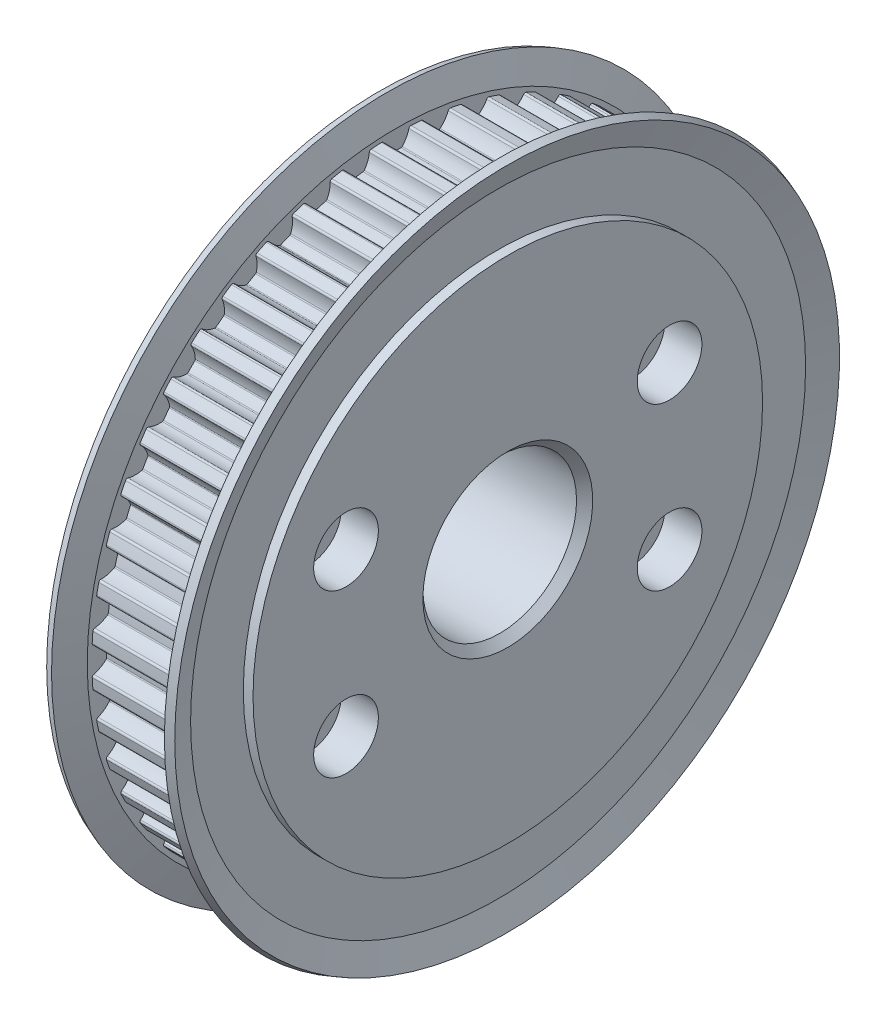
SolidWorks part; units mm, degrees
material "A7075"
ref_plane "Front Plane" through (0, 0, 0) normal (0, 0, 1) x (1, 0, 0)
ref_plane "Top Plane" through (0, 0, 0) normal (0, 1, 0) x (1, 0, 0)
ref_plane "Right Plane" through (0, 0, 0) normal (1, 0, 0) x (0, 0, -1)
sketch "Sketch1" plane through (0, 0, 0) normal (0, 0, 1) x (1, 0, 0)
  line L0 (0, 31.5) -> (0, 7.7)
  line L1 (0, 7.7) -> (0.2, 7.5)
  line L2 (0.2, 7.5) -> (27.8, 7.5)
  line L3 (27.8, 7.5) -> (28, 7.7)
  line L4 (28, 7.7) -> (28, 28.8)
  line L5 (28, 28.8) -> (27.8, 29)
  line L6 (27.8, 29) -> (16, 29)
  line L7 (16, 29) -> (16, 31.5)
  line L8 (16, 31.5) -> (14.8, 31.5)
  line L9 (14.8, 31.5) -> (14.8, 38.0191)
  line L10 (14.8, 38.0191) -> (15.9167, 41.0946)
  line L11 (15.9167, 41.0946) -> (14.9767, 41.4358)
  line L12 (14.9767, 41.4358) -> (13.8, 38.195)
  line L13 (13.8, 38.195) -> (2.2, 38.195)
  line L14 (2.2, 38.195) -> (1.0233, 41.4358)
  line L15 (1.0233, 41.4358) -> (0.0833, 41.0946)
  line L16 (0.0833, 41.0946) -> (1.2, 38.0191)
  line L17 (1.2, 38.0191) -> (1.2, 31.5)
  line L18 (1.2, 31.5) -> (0, 31.5)
  line L19 (28, 0) -> (0, 0) construction
revolve "Revolve1" add sketch "Sketch1" angle 360 about L19
sketch "Sketch2" plane through (0, 0, 0) normal (0, 0, 1) x (1, 0, 0)
  line L0 (16, 0) -> (16, 30)
  line L1 (16, 30) -> (28, 30)
  line L2 (28, 30) -> (28, 0)
  line L3 (28, 0) -> (16, 0)
  line L4 (28, 0) -> (16, 0) construction
revolve "Cut-Revolve1" cut sketch "Sketch2" angle 360 about L4
ref_plane "Plane1" through (2.2, 0, 0) normal (1, 0, 0) x (0, 0, -1)
sketch "Sketch3" plane through (2.2, 0, 0) normal (1, 0, 0) x (0, 0, -1)
  line L0 (-76.39, -76.39) -> (76.39, -76.39)
  line L1 (76.39, -76.39) -> (76.39, 76.39)
  line L2 (76.39, 76.39) -> (-76.39, 76.39)
  line L3 (-76.39, 76.39) -> (-76.39, -76.39)
  arc A0 (-37.5807, 1.8248) -> (-37.389, 1.5695) centre (-37.331, 1.8127) ccw
  arc A1 (-37.389, 1.5695) -> (-35.8722, 0.747) centre (-38.1589, -1.66) cw
  arc A2 (-35.8722, 0.747) -> (-35.81, 0.5986) centre (-36.01, 0.602) cw
  arc A3 (-35.81, 0.5986) -> (-35.81, -0.5986) centre (0, 0) ccw
  arc A4 (-35.81, -0.5986) -> (-35.8722, -0.747) centre (-36.01, -0.602) cw
  arc A5 (-35.8722, -0.747) -> (-37.389, -1.5695) centre (-38.1589, 1.66) cw
  arc A6 (-37.389, -1.5695) -> (-37.5807, -1.8248) centre (-37.331, -1.8127) ccw
  arc A7 (-37.5807, -1.8248) -> (-37.5444, -2.4608) centre (0, 0) ccw
  arc A8 (-37.5444, -2.4608) -> (-37.4974, -3.0961) centre (0, 0) ccw
  arc A9 (-37.4974, -3.0961) -> (-37.274, -3.3242) centre (-37.2482, -3.0755) ccw
  arc A10 (-37.274, -3.3242) -> (-35.6628, -3.9417) centre (-37.6158, -6.6265) cw
  arc A11 (-35.6628, -3.9417) -> (-35.5818, -4.0806) centre (-35.7805, -4.1034) cw
  arc A12 (-35.5818, -4.0806) -> (-35.4255, -5.2676) centre (0, 0) ccw
  arc A13 (-35.4255, -5.2676) -> (-35.4678, -5.4228) centre (-35.6233, -5.2971) cw
  arc A14 (-35.4678, -5.4228) -> (-36.8643, -6.4363) centre (-38.0491, -3.3349) cw
  arc A15 (-36.8643, -6.4363) -> (-37.021, -6.7145) centre (-36.775, -6.6698) ccw
  arc A16 (-37.021, -6.7145) -> (-36.902, -7.3403) centre (0, 0) ccw
  arc A17 (-36.902, -7.3403) -> (-36.7725, -7.964) centre (0, 0) ccw
  arc A18 (-36.7725, -7.964) -> (-36.5212, -8.161) centre (-36.5281, -7.9111) ccw
  arc A19 (-36.5212, -8.161) -> (-34.8432, -8.5629) centre (-36.429, -11.4797) cw
  arc A20 (-34.8432, -8.5629) -> (-34.7447, -8.6901) centre (-34.9388, -8.7386) cw
  arc A21 (-34.7447, -8.6901) -> (-34.4349, -9.8465) centre (0, 0) ccw
  arc A22 (-34.4349, -9.8465) -> (-34.4566, -10.0059) centre (-34.6272, -9.9015) cw
  arc A23 (-34.4566, -10.0059) -> (-35.7088, -11.193) centre (-37.2883, -8.2728) cw
  arc A24 (-35.7088, -11.193) -> (-35.8279, -11.4892) centre (-35.5898, -11.4129) ccw
  arc A25 (-35.8279, -11.4892) -> (-35.6282, -12.0942) centre (0, 0) ccw
  arc A26 (-35.6282, -12.0942) -> (-35.4184, -12.6956) centre (0, 0) ccw
  arc A27 (-35.4184, -12.6956) -> (-35.1435, -12.8581) centre (-35.183, -12.6113) ccw
  arc A28 (-35.1435, -12.8581) -> (-33.4275, -13.0376) centre (-34.619, -16.1364) cw
  arc A29 (-33.4275, -13.0376) -> (-33.3132, -13.1508) centre (-33.4992, -13.2243) cw
  arc A30 (-33.3132, -13.1508) -> (-32.855, -14.2569) centre (0, 0) ccw
  arc A31 (-32.855, -14.2569) -> (-32.8558, -14.4178) centre (-33.0385, -14.3366) cw
  arc A32 (-32.8558, -14.4178) -> (-33.9423, -15.7582) centre (-35.8895, -13.0691) cw
  arc A33 (-33.9423, -15.7582) -> (-34.0217, -16.0674) centre (-33.7957, -15.9607) ccw
  arc A34 (-34.0217, -16.0674) -> (-33.7448, -16.6411) centre (0, 0) ccw
  arc A35 (-33.7448, -16.6411) -> (-33.4583, -17.21) centre (0, 0) ccw
  arc A36 (-33.4583, -17.21) -> (-33.1646, -17.3353) centre (-33.2359, -17.0957) ccw
  arc A37 (-33.1646, -17.3353) -> (-31.4397, -17.2892) centre (-32.2166, -20.5171) cw
  arc A38 (-31.4397, -17.2892) -> (-31.3117, -17.3866) centre (-31.4865, -17.4837) cw
  arc A39 (-31.3117, -17.3866) -> (-30.7131, -18.4234) centre (0, 0) ccw
  arc A40 (-30.7131, -18.4234) -> (-30.6928, -18.583) centre (-30.8846, -18.5263) cw
  arc A41 (-30.6928, -18.583) -> (-31.5951, -20.0537) centre (-33.8766, -17.6419) cw
  arc A42 (-31.5951, -20.0537) -> (-31.6335, -20.3707) centre (-31.4233, -20.2353) ccw
  arc A43 (-31.6335, -20.3707) -> (-31.284, -20.9033) centre (0, 0) ccw
  arc A44 (-31.284, -20.9033) -> (-30.9257, -21.43) centre (0, 0) ccw
  arc A45 (-30.9257, -21.43) -> (-30.6181, -21.5158) centre (-30.7202, -21.2876) ccw
  arc A46 (-30.6181, -21.5158) -> (-28.9141, -21.245) centre (-29.263, -24.5466) cw
  arc A47 (-28.9141, -21.245) -> (-28.7744, -21.3248) centre (-28.9351, -21.4439) cw
  arc A48 (-28.7744, -21.3248) -> (-28.0456, -22.2747) centre (0, 0) ccw
  arc A49 (-28.0456, -22.2747) -> (-28.0046, -22.4302) centre (-28.2022, -22.399) cw
  arc A50 (-28.0046, -22.4302) -> (-28.7072, -24.0061) centre (-31.284, -21.9127) cw
  arc A51 (-28.7072, -24.0061) -> (-28.7039, -24.3254) centre (-28.5132, -24.1638) ccw
  arc A52 (-28.7039, -24.3254) -> (-28.288, -24.8079) centre (0, 0) ccw
  arc A53 (-28.288, -24.8079) -> (-27.8639, -25.2833) centre (0, 0) ccw
  arc A54 (-27.8639, -25.2833) -> (-27.5478, -25.3282) centre (-27.6788, -25.1153) ccw
  arc A55 (-27.5478, -25.3282) -> (-25.8937, -24.8373) centre (-25.8086, -28.1562) cw
  arc A56 (-25.8937, -24.8373) -> (-25.7448, -24.8982) centre (-25.8885, -25.0372) cw
  arc A57 (-25.7448, -24.8982) -> (-24.8982, -25.7448) centre (0, 0) ccw
  arc A58 (-24.8982, -25.7448) -> (-24.8373, -25.8937) centre (-25.0372, -25.8885) cw
  arc A59 (-24.8373, -25.8937) -> (-25.3282, -27.5478) centre (-28.1562, -25.8086) cw
  arc A60 (-25.3282, -27.5478) -> (-25.2833, -27.8639) centre (-25.1153, -27.6788) ccw
  arc A61 (-25.2833, -27.8639) -> (-24.8079, -28.288) centre (0, 0) ccw
  arc A62 (-24.8079, -28.288) -> (-24.3254, -28.7039) centre (0, 0) ccw
  arc A63 (-24.3254, -28.7039) -> (-24.0061, -28.7072) centre (-24.1638, -28.5132) ccw
  arc A64 (-24.0061, -28.7072) -> (-22.4302, -28.0046) centre (-21.9127, -31.284) cw
  arc A65 (-22.4302, -28.0046) -> (-22.2747, -28.0456) centre (-22.399, -28.2022) cw
  arc A66 (-22.2747, -28.0456) -> (-21.3248, -28.7744) centre (0, 0) ccw
  arc A67 (-21.3248, -28.7744) -> (-21.245, -28.9141) centre (-21.4439, -28.9351) cw
  arc A68 (-21.245, -28.9141) -> (-21.5158, -30.6181) centre (-24.5466, -29.263) cw
  arc A69 (-21.5158, -30.6181) -> (-21.43, -30.9257) centre (-21.2876, -30.7202) ccw
  arc A70 (-21.43, -30.9257) -> (-20.9033, -31.284) centre (0, 0) ccw
  arc A71 (-20.9033, -31.284) -> (-20.3707, -31.6335) centre (0, 0) ccw
  arc A72 (-20.3707, -31.6335) -> (-20.0537, -31.5951) centre (-20.2353, -31.4233) ccw
  arc A73 (-20.0537, -31.5951) -> (-18.583, -30.6928) centre (-17.6419, -33.8766) cw
  arc A74 (-18.583, -30.6928) -> (-18.4234, -30.7131) centre (-18.5263, -30.8846) cw
  arc A75 (-18.4234, -30.7131) -> (-17.3866, -31.3117) centre (0, 0) ccw
  arc A76 (-17.3866, -31.3117) -> (-17.2892, -31.4397) centre (-17.4837, -31.4865) cw
  arc A77 (-17.2892, -31.4397) -> (-17.3353, -33.1646) centre (-20.5171, -32.2166) cw
  arc A78 (-17.3353, -33.1646) -> (-17.21, -33.4583) centre (-17.0957, -33.2359) ccw
  arc A79 (-17.21, -33.4583) -> (-16.6411, -33.7448) centre (0, 0) ccw
  arc A80 (-16.6411, -33.7448) -> (-16.0674, -34.0217) centre (0, 0) ccw
  arc A81 (-16.0674, -34.0217) -> (-15.7582, -33.9423) centre (-15.9607, -33.7957) ccw
  arc A82 (-15.7582, -33.9423) -> (-14.4178, -32.8558) centre (-13.0691, -35.8895) cw
  arc A83 (-14.4178, -32.8558) -> (-14.2569, -32.855) centre (-14.3366, -33.0385) cw
  arc A84 (-14.2569, -32.855) -> (-13.1508, -33.3132) centre (0, 0) ccw
  arc A85 (-13.1508, -33.3132) -> (-13.0376, -33.4275) centre (-13.2243, -33.4992) cw
  arc A86 (-13.0376, -33.4275) -> (-12.8581, -35.1435) centre (-16.1364, -34.619) cw
  arc A87 (-12.8581, -35.1435) -> (-12.6956, -35.4184) centre (-12.6113, -35.183) ccw
  arc A88 (-12.6956, -35.4184) -> (-12.0942, -35.6282) centre (0, 0) ccw
  arc A89 (-12.0942, -35.6282) -> (-11.4892, -35.8279) centre (0, 0) ccw
  arc A90 (-11.4892, -35.8279) -> (-11.193, -35.7088) centre (-11.4129, -35.5898) ccw
  arc A91 (-11.193, -35.7088) -> (-10.0059, -34.4566) centre (-8.2728, -37.2883) cw
  arc A92 (-10.0059, -34.4566) -> (-9.8465, -34.4349) centre (-9.9015, -34.6272) cw
  arc A93 (-9.8465, -34.4349) -> (-8.6901, -34.7447) centre (0, 0) ccw
  arc A94 (-8.6901, -34.7447) -> (-8.5629, -34.8432) centre (-8.7386, -34.9388) cw
  arc A95 (-8.5629, -34.8432) -> (-8.161, -36.5212) centre (-11.4797, -36.429) cw
  arc A96 (-8.161, -36.5212) -> (-7.964, -36.7725) centre (-7.9111, -36.5281) ccw
  arc A97 (-7.964, -36.7725) -> (-7.3403, -36.902) centre (0, 0) ccw
  arc A98 (-7.3403, -36.902) -> (-6.7145, -37.021) centre (0, 0) ccw
  arc A99 (-6.7145, -37.021) -> (-6.4363, -36.8643) centre (-6.6698, -36.775) ccw
  arc A100 (-6.4363, -36.8643) -> (-5.4228, -35.4678) centre (-3.3349, -38.0491) cw
  arc A101 (-5.4228, -35.4678) -> (-5.2676, -35.4255) centre (-5.2971, -35.6233) cw
  arc A102 (-5.2676, -35.4255) -> (-4.0806, -35.5818) centre (0, 0) ccw
  arc A103 (-4.0806, -35.5818) -> (-3.9417, -35.6628) centre (-4.1034, -35.7805) cw
  arc A104 (-3.9417, -35.6628) -> (-3.3242, -37.274) centre (-6.6265, -37.6158) cw
  arc A105 (-3.3242, -37.274) -> (-3.0961, -37.4974) centre (-3.0755, -37.2482) ccw
  arc A106 (-3.0961, -37.4974) -> (-2.4608, -37.5444) centre (0, 0) ccw
  arc A107 (-2.4608, -37.5444) -> (-1.8248, -37.5807) centre (0, 0) ccw
  arc A108 (-1.8248, -37.5807) -> (-1.5695, -37.389) centre (-1.8127, -37.331) ccw
  arc A109 (-1.5695, -37.389) -> (-0.747, -35.8722) centre (1.66, -38.1589) cw
  arc A110 (-0.747, -35.8722) -> (-0.5986, -35.81) centre (-0.602, -36.01) cw
  arc A111 (-0.5986, -35.81) -> (0.5986, -35.81) centre (0, 0) ccw
  arc A112 (0.5986, -35.81) -> (0.747, -35.8722) centre (0.602, -36.01) cw
  arc A113 (0.747, -35.8722) -> (1.5695, -37.389) centre (-1.66, -38.1589) cw
  arc A114 (1.5695, -37.389) -> (1.8248, -37.5807) centre (1.8127, -37.331) ccw
  arc A115 (1.8248, -37.5807) -> (2.4608, -37.5444) centre (0, 0) ccw
  arc A116 (2.4608, -37.5444) -> (3.0961, -37.4974) centre (0, 0) ccw
  arc A117 (3.0961, -37.4974) -> (3.3242, -37.274) centre (3.0755, -37.2482) ccw
  arc A118 (3.3242, -37.274) -> (3.9417, -35.6628) centre (6.6265, -37.6158) cw
  arc A119 (3.9417, -35.6628) -> (4.0806, -35.5818) centre (4.1034, -35.7805) cw
  arc A120 (4.0806, -35.5818) -> (5.2676, -35.4255) centre (0, 0) ccw
  arc A121 (5.2676, -35.4255) -> (5.4228, -35.4678) centre (5.2971, -35.6233) cw
  arc A122 (5.4228, -35.4678) -> (6.4363, -36.8643) centre (3.3349, -38.0491) cw
  arc A123 (6.4363, -36.8643) -> (6.7145, -37.021) centre (6.6698, -36.775) ccw
  arc A124 (6.7145, -37.021) -> (7.3403, -36.902) centre (0, 0) ccw
  arc A125 (7.3403, -36.902) -> (7.964, -36.7725) centre (0, 0) ccw
  arc A126 (7.964, -36.7725) -> (8.161, -36.5212) centre (7.9111, -36.5281) ccw
  arc A127 (8.161, -36.5212) -> (8.5629, -34.8432) centre (11.4797, -36.429) cw
  arc A128 (8.5629, -34.8432) -> (8.6901, -34.7447) centre (8.7386, -34.9388) cw
  arc A129 (8.6901, -34.7447) -> (9.8465, -34.4349) centre (0, 0) ccw
  arc A130 (9.8465, -34.4349) -> (10.0059, -34.4566) centre (9.9015, -34.6272) cw
  arc A131 (10.0059, -34.4566) -> (11.193, -35.7088) centre (8.2728, -37.2883) cw
  arc A132 (11.193, -35.7088) -> (11.4892, -35.8279) centre (11.4129, -35.5898) ccw
  arc A133 (11.4892, -35.8279) -> (12.0942, -35.6282) centre (0, 0) ccw
  arc A134 (12.0942, -35.6282) -> (12.6956, -35.4184) centre (0, 0) ccw
  arc A135 (12.6956, -35.4184) -> (12.8581, -35.1435) centre (12.6113, -35.183) ccw
  arc A136 (12.8581, -35.1435) -> (13.0376, -33.4275) centre (16.1364, -34.619) cw
  arc A137 (13.0376, -33.4275) -> (13.1508, -33.3132) centre (13.2243, -33.4992) cw
  arc A138 (13.1508, -33.3132) -> (14.2569, -32.855) centre (0, 0) ccw
  arc A139 (14.2569, -32.855) -> (14.4178, -32.8558) centre (14.3366, -33.0385) cw
  arc A140 (14.4178, -32.8558) -> (15.7582, -33.9423) centre (13.0691, -35.8895) cw
  arc A141 (15.7582, -33.9423) -> (16.0674, -34.0217) centre (15.9607, -33.7957) ccw
  arc A142 (16.0674, -34.0217) -> (16.6411, -33.7448) centre (0, 0) ccw
  arc A143 (16.6411, -33.7448) -> (17.21, -33.4583) centre (0, 0) ccw
  arc A144 (17.21, -33.4583) -> (17.3353, -33.1646) centre (17.0957, -33.2359) ccw
  arc A145 (17.3353, -33.1646) -> (17.2892, -31.4397) centre (20.5171, -32.2166) cw
  arc A146 (17.2892, -31.4397) -> (17.3866, -31.3117) centre (17.4837, -31.4865) cw
  arc A147 (17.3866, -31.3117) -> (18.4234, -30.7131) centre (0, 0) ccw
  arc A148 (18.4234, -30.7131) -> (18.583, -30.6928) centre (18.5263, -30.8846) cw
  arc A149 (18.583, -30.6928) -> (20.0537, -31.5951) centre (17.6419, -33.8766) cw
  arc A150 (20.0537, -31.5951) -> (20.3707, -31.6335) centre (20.2353, -31.4233) ccw
  arc A151 (20.3707, -31.6335) -> (20.9033, -31.284) centre (0, 0) ccw
  arc A152 (20.9033, -31.284) -> (21.43, -30.9257) centre (0, 0) ccw
  arc A153 (21.43, -30.9257) -> (21.5158, -30.6181) centre (21.2876, -30.7202) ccw
  arc A154 (21.5158, -30.6181) -> (21.245, -28.9141) centre (24.5466, -29.263) cw
  arc A155 (21.245, -28.9141) -> (21.3248, -28.7744) centre (21.4439, -28.9351) cw
  arc A156 (21.3248, -28.7744) -> (22.2747, -28.0456) centre (0, 0) ccw
  arc A157 (22.2747, -28.0456) -> (22.4302, -28.0046) centre (22.399, -28.2022) cw
  arc A158 (22.4302, -28.0046) -> (24.0061, -28.7072) centre (21.9127, -31.284) cw
  arc A159 (24.0061, -28.7072) -> (24.3254, -28.7039) centre (24.1638, -28.5132) ccw
  arc A160 (24.3254, -28.7039) -> (24.8079, -28.288) centre (0, 0) ccw
  arc A161 (24.8079, -28.288) -> (25.2833, -27.8639) centre (0, 0) ccw
  arc A162 (25.2833, -27.8639) -> (25.3282, -27.5478) centre (25.1153, -27.6788) ccw
  arc A163 (25.3282, -27.5478) -> (24.8373, -25.8937) centre (28.1562, -25.8086) cw
  arc A164 (24.8373, -25.8937) -> (24.8982, -25.7448) centre (25.0372, -25.8885) cw
  arc A165 (24.8982, -25.7448) -> (25.7448, -24.8982) centre (0, 0) ccw
  arc A166 (25.7448, -24.8982) -> (25.8937, -24.8373) centre (25.8885, -25.0372) cw
  arc A167 (25.8937, -24.8373) -> (27.5478, -25.3282) centre (25.8086, -28.1562) cw
  arc A168 (27.5478, -25.3282) -> (27.8639, -25.2833) centre (27.6788, -25.1153) ccw
  arc A169 (27.8639, -25.2833) -> (28.288, -24.8079) centre (0, 0) ccw
  arc A170 (28.288, -24.8079) -> (28.7039, -24.3254) centre (0, 0) ccw
  arc A171 (28.7039, -24.3254) -> (28.7072, -24.0061) centre (28.5132, -24.1638) ccw
  arc A172 (28.7072, -24.0061) -> (28.0046, -22.4302) centre (31.284, -21.9127) cw
  arc A173 (28.0046, -22.4302) -> (28.0456, -22.2747) centre (28.2022, -22.399) cw
  arc A174 (28.0456, -22.2747) -> (28.7744, -21.3248) centre (0, 0) ccw
  arc A175 (28.7744, -21.3248) -> (28.9141, -21.245) centre (28.9351, -21.4439) cw
  arc A176 (28.9141, -21.245) -> (30.6181, -21.5158) centre (29.263, -24.5466) cw
  arc A177 (30.6181, -21.5158) -> (30.9257, -21.43) centre (30.7202, -21.2876) ccw
  arc A178 (30.9257, -21.43) -> (31.284, -20.9033) centre (0, 0) ccw
  arc A179 (31.284, -20.9033) -> (31.6335, -20.3707) centre (0, 0) ccw
  arc A180 (31.6335, -20.3707) -> (31.5951, -20.0537) centre (31.4233, -20.2353) ccw
  arc A181 (31.5951, -20.0537) -> (30.6928, -18.583) centre (33.8766, -17.6419) cw
  arc A182 (30.6928, -18.583) -> (30.7131, -18.4234) centre (30.8846, -18.5263) cw
  arc A183 (30.7131, -18.4234) -> (31.3117, -17.3866) centre (0, 0) ccw
  arc A184 (31.3117, -17.3866) -> (31.4397, -17.2892) centre (31.4865, -17.4837) cw
  arc A185 (31.4397, -17.2892) -> (33.1646, -17.3353) centre (32.2166, -20.5171) cw
  arc A186 (33.1646, -17.3353) -> (33.4583, -17.21) centre (33.2359, -17.0957) ccw
  arc A187 (33.4583, -17.21) -> (33.7448, -16.6411) centre (0, 0) ccw
  arc A188 (33.7448, -16.6411) -> (34.0217, -16.0674) centre (0, 0) ccw
  arc A189 (34.0217, -16.0674) -> (33.9423, -15.7582) centre (33.7957, -15.9607) ccw
  arc A190 (33.9423, -15.7582) -> (32.8558, -14.4178) centre (35.8895, -13.0691) cw
  arc A191 (32.8558, -14.4178) -> (32.855, -14.2569) centre (33.0385, -14.3366) cw
  arc A192 (32.855, -14.2569) -> (33.3132, -13.1508) centre (0, 0) ccw
  arc A193 (33.3132, -13.1508) -> (33.4275, -13.0376) centre (33.4992, -13.2243) cw
  arc A194 (33.4275, -13.0376) -> (35.1435, -12.8581) centre (34.619, -16.1364) cw
  arc A195 (35.1435, -12.8581) -> (35.4184, -12.6956) centre (35.183, -12.6113) ccw
  arc A196 (35.4184, -12.6956) -> (35.6282, -12.0942) centre (0, 0) ccw
  arc A197 (35.6282, -12.0942) -> (35.8279, -11.4892) centre (0, 0) ccw
  arc A198 (35.8279, -11.4892) -> (35.7088, -11.193) centre (35.5898, -11.4129) ccw
  arc A199 (35.7088, -11.193) -> (34.4566, -10.0059) centre (37.2883, -8.2728) cw
  arc A200 (34.4566, -10.0059) -> (34.4349, -9.8465) centre (34.6272, -9.9015) cw
  arc A201 (34.4349, -9.8465) -> (34.7447, -8.6901) centre (0, 0) ccw
  arc A202 (34.7447, -8.6901) -> (34.8432, -8.5629) centre (34.9388, -8.7386) cw
  arc A203 (34.8432, -8.5629) -> (36.5212, -8.161) centre (36.429, -11.4797) cw
  arc A204 (36.5212, -8.161) -> (36.7725, -7.964) centre (36.5281, -7.9111) ccw
  arc A205 (36.7725, -7.964) -> (36.902, -7.3403) centre (0, 0) ccw
  arc A206 (36.902, -7.3403) -> (37.021, -6.7145) centre (0, 0) ccw
  arc A207 (37.021, -6.7145) -> (36.8643, -6.4363) centre (36.775, -6.6698) ccw
  arc A208 (36.8643, -6.4363) -> (35.4678, -5.4228) centre (38.0491, -3.3349) cw
  arc A209 (35.4678, -5.4228) -> (35.4255, -5.2676) centre (35.6233, -5.2971) cw
  arc A210 (35.4255, -5.2676) -> (35.5818, -4.0806) centre (0, 0) ccw
  arc A211 (35.5818, -4.0806) -> (35.6628, -3.9417) centre (35.7805, -4.1034) cw
  arc A212 (35.6628, -3.9417) -> (37.274, -3.3242) centre (37.6158, -6.6265) cw
  arc A213 (37.274, -3.3242) -> (37.4974, -3.0961) centre (37.2482, -3.0755) ccw
  arc A214 (37.4974, -3.0961) -> (37.5444, -2.4608) centre (0, 0) ccw
  arc A215 (37.5444, -2.4608) -> (37.5807, -1.8248) centre (0, 0) ccw
  arc A216 (37.5807, -1.8248) -> (37.389, -1.5695) centre (37.331, -1.8127) ccw
  arc A217 (37.389, -1.5695) -> (35.8722, -0.747) centre (38.1589, 1.66) cw
  arc A218 (35.8722, -0.747) -> (35.81, -0.5986) centre (36.01, -0.602) cw
  arc A219 (35.81, -0.5986) -> (35.81, 0.5986) centre (0, 0) ccw
  arc A220 (35.81, 0.5986) -> (35.8722, 0.747) centre (36.01, 0.602) cw
  arc A221 (35.8722, 0.747) -> (37.389, 1.5695) centre (38.1589, -1.66) cw
  arc A222 (37.389, 1.5695) -> (37.5807, 1.8248) centre (37.331, 1.8127) ccw
  arc A223 (37.5807, 1.8248) -> (37.5444, 2.4608) centre (0, 0) ccw
  arc A224 (37.5444, 2.4608) -> (37.4974, 3.0961) centre (0, 0) ccw
  arc A225 (37.4974, 3.0961) -> (37.274, 3.3242) centre (37.2482, 3.0755) ccw
  arc A226 (37.274, 3.3242) -> (35.6628, 3.9417) centre (37.6158, 6.6265) cw
  arc A227 (35.6628, 3.9417) -> (35.5818, 4.0806) centre (35.7805, 4.1034) cw
  arc A228 (35.5818, 4.0806) -> (35.4255, 5.2676) centre (0, 0) ccw
  arc A229 (35.4255, 5.2676) -> (35.4678, 5.4228) centre (35.6233, 5.2971) cw
  arc A230 (35.4678, 5.4228) -> (36.8643, 6.4363) centre (38.0491, 3.3349) cw
  arc A231 (36.8643, 6.4363) -> (37.021, 6.7145) centre (36.775, 6.6698) ccw
  arc A232 (37.021, 6.7145) -> (36.902, 7.3403) centre (0, 0) ccw
  arc A233 (36.902, 7.3403) -> (36.7725, 7.964) centre (0, 0) ccw
  arc A234 (36.7725, 7.964) -> (36.5212, 8.161) centre (36.5281, 7.9111) ccw
  arc A235 (36.5212, 8.161) -> (34.8432, 8.5629) centre (36.429, 11.4797) cw
  arc A236 (34.8432, 8.5629) -> (34.7447, 8.6901) centre (34.9388, 8.7386) cw
  arc A237 (34.7447, 8.6901) -> (34.4349, 9.8465) centre (0, 0) ccw
  arc A238 (34.4349, 9.8465) -> (34.4566, 10.0059) centre (34.6272, 9.9015) cw
  arc A239 (34.4566, 10.0059) -> (35.7088, 11.193) centre (37.2883, 8.2728) cw
  arc A240 (35.7088, 11.193) -> (35.8279, 11.4892) centre (35.5898, 11.4129) ccw
  arc A241 (35.8279, 11.4892) -> (35.6282, 12.0942) centre (0, 0) ccw
  arc A242 (35.6282, 12.0942) -> (35.4184, 12.6956) centre (0, 0) ccw
  arc A243 (35.4184, 12.6956) -> (35.1435, 12.8581) centre (35.183, 12.6113) ccw
  arc A244 (35.1435, 12.8581) -> (33.4275, 13.0376) centre (34.619, 16.1364) cw
  arc A245 (33.4275, 13.0376) -> (33.3132, 13.1508) centre (33.4992, 13.2243) cw
  arc A246 (33.3132, 13.1508) -> (32.855, 14.2569) centre (0, 0) ccw
  arc A247 (32.855, 14.2569) -> (32.8558, 14.4178) centre (33.0385, 14.3366) cw
  arc A248 (32.8558, 14.4178) -> (33.9423, 15.7582) centre (35.8895, 13.0691) cw
  arc A249 (33.9423, 15.7582) -> (34.0217, 16.0674) centre (33.7957, 15.9607) ccw
  arc A250 (34.0217, 16.0674) -> (33.7448, 16.6411) centre (0, 0) ccw
  arc A251 (33.7448, 16.6411) -> (33.4583, 17.21) centre (0, 0) ccw
  arc A252 (33.4583, 17.21) -> (33.1646, 17.3353) centre (33.2359, 17.0957) ccw
  arc A253 (33.1646, 17.3353) -> (31.4397, 17.2892) centre (32.2166, 20.5171) cw
  arc A254 (31.4397, 17.2892) -> (31.3117, 17.3866) centre (31.4865, 17.4837) cw
  arc A255 (31.3117, 17.3866) -> (30.7131, 18.4234) centre (0, 0) ccw
  arc A256 (30.7131, 18.4234) -> (30.6928, 18.583) centre (30.8846, 18.5263) cw
  arc A257 (30.6928, 18.583) -> (31.5951, 20.0537) centre (33.8766, 17.6419) cw
  arc A258 (31.5951, 20.0537) -> (31.6335, 20.3707) centre (31.4233, 20.2353) ccw
  arc A259 (31.6335, 20.3707) -> (31.284, 20.9033) centre (0, 0) ccw
  arc A260 (31.284, 20.9033) -> (30.9257, 21.43) centre (0, 0) ccw
  arc A261 (30.9257, 21.43) -> (30.6181, 21.5158) centre (30.7202, 21.2876) ccw
  arc A262 (30.6181, 21.5158) -> (28.9141, 21.245) centre (29.263, 24.5466) cw
  arc A263 (28.9141, 21.245) -> (28.7744, 21.3248) centre (28.9351, 21.4439) cw
  arc A264 (28.7744, 21.3248) -> (28.0456, 22.2747) centre (0, 0) ccw
  arc A265 (28.0456, 22.2747) -> (28.0046, 22.4302) centre (28.2022, 22.399) cw
  arc A266 (28.0046, 22.4302) -> (28.7072, 24.0061) centre (31.284, 21.9127) cw
  arc A267 (28.7072, 24.0061) -> (28.7039, 24.3254) centre (28.5132, 24.1638) ccw
  arc A268 (28.7039, 24.3254) -> (28.288, 24.8079) centre (0, 0) ccw
  arc A269 (28.288, 24.8079) -> (27.8639, 25.2833) centre (0, 0) ccw
  arc A270 (27.8639, 25.2833) -> (27.5478, 25.3282) centre (27.6788, 25.1153) ccw
  arc A271 (27.5478, 25.3282) -> (25.8937, 24.8373) centre (25.8086, 28.1562) cw
  arc A272 (25.8937, 24.8373) -> (25.7448, 24.8982) centre (25.8885, 25.0372) cw
  arc A273 (25.7448, 24.8982) -> (24.8982, 25.7448) centre (0, 0) ccw
  arc A274 (24.8982, 25.7448) -> (24.8373, 25.8937) centre (25.0372, 25.8885) cw
  arc A275 (24.8373, 25.8937) -> (25.3282, 27.5478) centre (28.1562, 25.8086) cw
  arc A276 (25.3282, 27.5478) -> (25.2833, 27.8639) centre (25.1153, 27.6788) ccw
  arc A277 (25.2833, 27.8639) -> (24.8079, 28.288) centre (0, 0) ccw
  arc A278 (24.8079, 28.288) -> (24.3254, 28.7039) centre (0, 0) ccw
  arc A279 (24.3254, 28.7039) -> (24.0061, 28.7072) centre (24.1638, 28.5132) ccw
  arc A280 (24.0061, 28.7072) -> (22.4302, 28.0046) centre (21.9127, 31.284) cw
  arc A281 (22.4302, 28.0046) -> (22.2747, 28.0456) centre (22.399, 28.2022) cw
  arc A282 (22.2747, 28.0456) -> (21.3248, 28.7744) centre (0, 0) ccw
  arc A283 (21.3248, 28.7744) -> (21.245, 28.9141) centre (21.4439, 28.9351) cw
  arc A284 (21.245, 28.9141) -> (21.5158, 30.6181) centre (24.5466, 29.263) cw
  arc A285 (21.5158, 30.6181) -> (21.43, 30.9257) centre (21.2876, 30.7202) ccw
  arc A286 (21.43, 30.9257) -> (20.9033, 31.284) centre (0, 0) ccw
  arc A287 (20.9033, 31.284) -> (20.3707, 31.6335) centre (0, 0) ccw
  arc A288 (20.3707, 31.6335) -> (20.0537, 31.5951) centre (20.2353, 31.4233) ccw
  arc A289 (20.0537, 31.5951) -> (18.583, 30.6928) centre (17.6419, 33.8766) cw
  arc A290 (18.583, 30.6928) -> (18.4234, 30.7131) centre (18.5263, 30.8846) cw
  arc A291 (18.4234, 30.7131) -> (17.3866, 31.3117) centre (0, 0) ccw
  arc A292 (17.3866, 31.3117) -> (17.2892, 31.4397) centre (17.4837, 31.4865) cw
  arc A293 (17.2892, 31.4397) -> (17.3353, 33.1646) centre (20.5171, 32.2166) cw
  arc A294 (17.3353, 33.1646) -> (17.21, 33.4583) centre (17.0957, 33.2359) ccw
  arc A295 (17.21, 33.4583) -> (16.6411, 33.7448) centre (0, 0) ccw
  arc A296 (16.6411, 33.7448) -> (16.0674, 34.0217) centre (0, 0) ccw
  arc A297 (16.0674, 34.0217) -> (15.7582, 33.9423) centre (15.9607, 33.7957) ccw
  arc A298 (15.7582, 33.9423) -> (14.4178, 32.8558) centre (13.0691, 35.8895) cw
  arc A299 (14.4178, 32.8558) -> (14.2569, 32.855) centre (14.3366, 33.0385) cw
  arc A300 (14.2569, 32.855) -> (13.1508, 33.3132) centre (0, 0) ccw
  arc A301 (13.1508, 33.3132) -> (13.0376, 33.4275) centre (13.2243, 33.4992) cw
  arc A302 (13.0376, 33.4275) -> (12.8581, 35.1435) centre (16.1364, 34.619) cw
  arc A303 (12.8581, 35.1435) -> (12.6956, 35.4184) centre (12.6113, 35.183) ccw
  arc A304 (12.6956, 35.4184) -> (12.0942, 35.6282) centre (0, 0) ccw
  arc A305 (12.0942, 35.6282) -> (11.4892, 35.8279) centre (0, 0) ccw
  arc A306 (11.4892, 35.8279) -> (11.193, 35.7088) centre (11.4129, 35.5898) ccw
  arc A307 (11.193, 35.7088) -> (10.0059, 34.4566) centre (8.2728, 37.2883) cw
  arc A308 (10.0059, 34.4566) -> (9.8465, 34.4349) centre (9.9015, 34.6272) cw
  arc A309 (9.8465, 34.4349) -> (8.6901, 34.7447) centre (0, 0) ccw
  arc A310 (8.6901, 34.7447) -> (8.5629, 34.8432) centre (8.7386, 34.9388) cw
  arc A311 (8.5629, 34.8432) -> (8.161, 36.5212) centre (11.4797, 36.429) cw
  arc A312 (8.161, 36.5212) -> (7.964, 36.7725) centre (7.9111, 36.5281) ccw
  arc A313 (7.964, 36.7725) -> (7.3403, 36.902) centre (0, 0) ccw
  arc A314 (7.3403, 36.902) -> (6.7145, 37.021) centre (0, 0) ccw
  arc A315 (6.7145, 37.021) -> (6.4363, 36.8643) centre (6.6698, 36.775) ccw
  arc A316 (6.4363, 36.8643) -> (5.4228, 35.4678) centre (3.3349, 38.0491) cw
  arc A317 (5.4228, 35.4678) -> (5.2676, 35.4255) centre (5.2971, 35.6233) cw
  arc A318 (5.2676, 35.4255) -> (4.0806, 35.5818) centre (0, 0) ccw
  arc A319 (4.0806, 35.5818) -> (3.9417, 35.6628) centre (4.1034, 35.7805) cw
  arc A320 (3.9417, 35.6628) -> (3.3242, 37.274) centre (6.6265, 37.6158) cw
  arc A321 (3.3242, 37.274) -> (3.0961, 37.4974) centre (3.0755, 37.2482) ccw
  arc A322 (3.0961, 37.4974) -> (2.4608, 37.5444) centre (0, 0) ccw
  arc A323 (2.4608, 37.5444) -> (1.8248, 37.5807) centre (0, 0) ccw
  arc A324 (1.8248, 37.5807) -> (1.5695, 37.389) centre (1.8127, 37.331) ccw
  arc A325 (1.5695, 37.389) -> (0.747, 35.8722) centre (-1.66, 38.1589) cw
  arc A326 (0.747, 35.8722) -> (0.5986, 35.81) centre (0.602, 36.01) cw
  arc A327 (0.5986, 35.81) -> (-0.5986, 35.81) centre (0, 0) ccw
  arc A328 (-0.5986, 35.81) -> (-0.747, 35.8722) centre (-0.602, 36.01) cw
  arc A329 (-0.747, 35.8722) -> (-1.5695, 37.389) centre (1.66, 38.1589) cw
  arc A330 (-1.5695, 37.389) -> (-1.8248, 37.5807) centre (-1.8127, 37.331) ccw
  arc A331 (-1.8248, 37.5807) -> (-2.4608, 37.5444) centre (0, 0) ccw
  arc A332 (-2.4608, 37.5444) -> (-3.0961, 37.4974) centre (0, 0) ccw
  arc A333 (-3.0961, 37.4974) -> (-3.3242, 37.274) centre (-3.0755, 37.2482) ccw
  arc A334 (-3.3242, 37.274) -> (-3.9417, 35.6628) centre (-6.6265, 37.6158) cw
  arc A335 (-3.9417, 35.6628) -> (-4.0806, 35.5818) centre (-4.1034, 35.7805) cw
  arc A336 (-4.0806, 35.5818) -> (-5.2676, 35.4255) centre (0, 0) ccw
  arc A337 (-5.2676, 35.4255) -> (-5.4228, 35.4678) centre (-5.2971, 35.6233) cw
  arc A338 (-5.4228, 35.4678) -> (-6.4363, 36.8643) centre (-3.3349, 38.0491) cw
  arc A339 (-6.4363, 36.8643) -> (-6.7145, 37.021) centre (-6.6698, 36.775) ccw
  arc A340 (-6.7145, 37.021) -> (-7.3403, 36.902) centre (0, 0) ccw
  arc A341 (-7.3403, 36.902) -> (-7.964, 36.7725) centre (0, 0) ccw
  arc A342 (-7.964, 36.7725) -> (-8.161, 36.5212) centre (-7.9111, 36.5281) ccw
  arc A343 (-8.161, 36.5212) -> (-8.5629, 34.8432) centre (-11.4797, 36.429) cw
  arc A344 (-8.5629, 34.8432) -> (-8.6901, 34.7447) centre (-8.7386, 34.9388) cw
  arc A345 (-8.6901, 34.7447) -> (-9.8465, 34.4349) centre (0, 0) ccw
  arc A346 (-9.8465, 34.4349) -> (-10.0059, 34.4566) centre (-9.9015, 34.6272) cw
  arc A347 (-10.0059, 34.4566) -> (-11.193, 35.7088) centre (-8.2728, 37.2883) cw
  arc A348 (-11.193, 35.7088) -> (-11.4892, 35.8279) centre (-11.4129, 35.5898) ccw
  arc A349 (-11.4892, 35.8279) -> (-12.0942, 35.6282) centre (0, 0) ccw
  arc A350 (-12.0942, 35.6282) -> (-12.6956, 35.4184) centre (0, 0) ccw
  arc A351 (-12.6956, 35.4184) -> (-12.8581, 35.1435) centre (-12.6113, 35.183) ccw
  arc A352 (-12.8581, 35.1435) -> (-13.0376, 33.4275) centre (-16.1364, 34.619) cw
  arc A353 (-13.0376, 33.4275) -> (-13.1508, 33.3132) centre (-13.2243, 33.4992) cw
  arc A354 (-13.1508, 33.3132) -> (-14.2569, 32.855) centre (0, 0) ccw
  arc A355 (-14.2569, 32.855) -> (-14.4178, 32.8558) centre (-14.3366, 33.0385) cw
  arc A356 (-14.4178, 32.8558) -> (-15.7582, 33.9423) centre (-13.0691, 35.8895) cw
  arc A357 (-15.7582, 33.9423) -> (-16.0674, 34.0217) centre (-15.9607, 33.7957) ccw
  arc A358 (-16.0674, 34.0217) -> (-16.6411, 33.7448) centre (0, 0) ccw
  arc A359 (-16.6411, 33.7448) -> (-17.21, 33.4583) centre (0, 0) ccw
  arc A360 (-17.21, 33.4583) -> (-17.3353, 33.1646) centre (-17.0957, 33.2359) ccw
  arc A361 (-17.3353, 33.1646) -> (-17.2892, 31.4397) centre (-20.5171, 32.2166) cw
  arc A362 (-17.2892, 31.4397) -> (-17.3866, 31.3117) centre (-17.4837, 31.4865) cw
  arc A363 (-17.3866, 31.3117) -> (-18.4234, 30.7131) centre (0, 0) ccw
  arc A364 (-18.4234, 30.7131) -> (-18.583, 30.6928) centre (-18.5263, 30.8846) cw
  arc A365 (-18.583, 30.6928) -> (-20.0537, 31.5951) centre (-17.6419, 33.8766) cw
  arc A366 (-20.0537, 31.5951) -> (-20.3707, 31.6335) centre (-20.2353, 31.4233) ccw
  arc A367 (-20.3707, 31.6335) -> (-20.9033, 31.284) centre (0, 0) ccw
  arc A368 (-20.9033, 31.284) -> (-21.43, 30.9257) centre (0, 0) ccw
  arc A369 (-21.43, 30.9257) -> (-21.5158, 30.6181) centre (-21.2876, 30.7202) ccw
  arc A370 (-21.5158, 30.6181) -> (-21.245, 28.9141) centre (-24.5466, 29.263) cw
  arc A371 (-21.245, 28.9141) -> (-21.3248, 28.7744) centre (-21.4439, 28.9351) cw
  arc A372 (-21.3248, 28.7744) -> (-22.2747, 28.0456) centre (0, 0) ccw
  arc A373 (-22.2747, 28.0456) -> (-22.4302, 28.0046) centre (-22.399, 28.2022) cw
  arc A374 (-22.4302, 28.0046) -> (-24.0061, 28.7072) centre (-21.9127, 31.284) cw
  arc A375 (-24.0061, 28.7072) -> (-24.3254, 28.7039) centre (-24.1638, 28.5132) ccw
  arc A376 (-24.3254, 28.7039) -> (-24.8079, 28.288) centre (0, 0) ccw
  arc A377 (-24.8079, 28.288) -> (-25.2833, 27.8639) centre (0, 0) ccw
  arc A378 (-25.2833, 27.8639) -> (-25.3282, 27.5478) centre (-25.1153, 27.6788) ccw
  arc A379 (-25.3282, 27.5478) -> (-24.8373, 25.8937) centre (-28.1562, 25.8086) cw
  arc A380 (-24.8373, 25.8937) -> (-24.8982, 25.7448) centre (-25.0372, 25.8885) cw
  arc A381 (-24.8982, 25.7448) -> (-25.7448, 24.8982) centre (0, 0) ccw
  arc A382 (-25.7448, 24.8982) -> (-25.8937, 24.8373) centre (-25.8885, 25.0372) cw
  arc A383 (-25.8937, 24.8373) -> (-27.5478, 25.3282) centre (-25.8086, 28.1562) cw
  arc A384 (-27.5478, 25.3282) -> (-27.8639, 25.2833) centre (-27.6788, 25.1153) ccw
  arc A385 (-27.8639, 25.2833) -> (-28.288, 24.8079) centre (0, 0) ccw
  arc A386 (-28.288, 24.8079) -> (-28.7039, 24.3254) centre (0, 0) ccw
  arc A387 (-28.7039, 24.3254) -> (-28.7072, 24.0061) centre (-28.5132, 24.1638) ccw
  arc A388 (-28.7072, 24.0061) -> (-28.0046, 22.4302) centre (-31.284, 21.9127) cw
  arc A389 (-28.0046, 22.4302) -> (-28.0456, 22.2747) centre (-28.2022, 22.399) cw
  arc A390 (-28.0456, 22.2747) -> (-28.7744, 21.3248) centre (0, 0) ccw
  arc A391 (-28.7744, 21.3248) -> (-28.9141, 21.245) centre (-28.9351, 21.4439) cw
  arc A392 (-28.9141, 21.245) -> (-30.6181, 21.5158) centre (-29.263, 24.5466) cw
  arc A393 (-30.6181, 21.5158) -> (-30.9257, 21.43) centre (-30.7202, 21.2876) ccw
  arc A394 (-30.9257, 21.43) -> (-31.284, 20.9033) centre (0, 0) ccw
  arc A395 (-31.284, 20.9033) -> (-31.6335, 20.3707) centre (0, 0) ccw
  arc A396 (-31.6335, 20.3707) -> (-31.5951, 20.0537) centre (-31.4233, 20.2353) ccw
  arc A397 (-31.5951, 20.0537) -> (-30.6928, 18.583) centre (-33.8766, 17.6419) cw
  arc A398 (-30.6928, 18.583) -> (-30.7131, 18.4234) centre (-30.8846, 18.5263) cw
  arc A399 (-30.7131, 18.4234) -> (-31.3117, 17.3866) centre (0, 0) ccw
  arc A400 (-31.3117, 17.3866) -> (-31.4397, 17.2892) centre (-31.4865, 17.4837) cw
  arc A401 (-31.4397, 17.2892) -> (-33.1646, 17.3353) centre (-32.2166, 20.5171) cw
  arc A402 (-33.1646, 17.3353) -> (-33.4583, 17.21) centre (-33.2359, 17.0957) ccw
  arc A403 (-33.4583, 17.21) -> (-33.7448, 16.6411) centre (0, 0) ccw
  arc A404 (-33.7448, 16.6411) -> (-34.0217, 16.0674) centre (0, 0) ccw
  arc A405 (-34.0217, 16.0674) -> (-33.9423, 15.7582) centre (-33.7957, 15.9607) ccw
  arc A406 (-33.9423, 15.7582) -> (-32.8558, 14.4178) centre (-35.8895, 13.0691) cw
  arc A407 (-32.8558, 14.4178) -> (-32.855, 14.2569) centre (-33.0385, 14.3366) cw
  arc A408 (-32.855, 14.2569) -> (-33.3132, 13.1508) centre (0, 0) ccw
  arc A409 (-33.3132, 13.1508) -> (-33.4275, 13.0376) centre (-33.4992, 13.2243) cw
  arc A410 (-33.4275, 13.0376) -> (-35.1435, 12.8581) centre (-34.619, 16.1364) cw
  arc A411 (-35.1435, 12.8581) -> (-35.4184, 12.6956) centre (-35.183, 12.6113) ccw
  arc A412 (-35.4184, 12.6956) -> (-35.6282, 12.0942) centre (0, 0) ccw
  arc A413 (-35.6282, 12.0942) -> (-35.8279, 11.4892) centre (0, 0) ccw
  arc A414 (-35.8279, 11.4892) -> (-35.7088, 11.193) centre (-35.5898, 11.4129) ccw
  arc A415 (-35.7088, 11.193) -> (-34.4566, 10.0059) centre (-37.2883, 8.2728) cw
  arc A416 (-34.4566, 10.0059) -> (-34.4349, 9.8465) centre (-34.6272, 9.9015) cw
  arc A417 (-34.4349, 9.8465) -> (-34.7447, 8.6901) centre (0, 0) ccw
  arc A418 (-34.7447, 8.6901) -> (-34.8432, 8.5629) centre (-34.9388, 8.7386) cw
  arc A419 (-34.8432, 8.5629) -> (-36.5212, 8.161) centre (-36.429, 11.4797) cw
  arc A420 (-36.5212, 8.161) -> (-36.7725, 7.964) centre (-36.5281, 7.9111) ccw
  arc A421 (-36.7725, 7.964) -> (-36.902, 7.3403) centre (0, 0) ccw
  arc A422 (-36.902, 7.3403) -> (-37.021, 6.7145) centre (0, 0) ccw
  arc A423 (-37.021, 6.7145) -> (-36.8643, 6.4363) centre (-36.775, 6.6698) ccw
  arc A424 (-36.8643, 6.4363) -> (-35.4678, 5.4228) centre (-38.0491, 3.3349) cw
  arc A425 (-35.4678, 5.4228) -> (-35.4255, 5.2676) centre (-35.6233, 5.2971) cw
  arc A426 (-35.4255, 5.2676) -> (-35.5818, 4.0806) centre (0, 0) ccw
  arc A427 (-35.5818, 4.0806) -> (-35.6628, 3.9417) centre (-35.7805, 4.1034) cw
  arc A428 (-35.6628, 3.9417) -> (-37.274, 3.3242) centre (-37.6158, 6.6265) cw
  arc A429 (-37.274, 3.3242) -> (-37.4974, 3.0961) centre (-37.2482, 3.0755) ccw
  arc A430 (-37.4974, 3.0961) -> (-37.5444, 2.4608) centre (0, 0) ccw
  arc A431 (-37.5444, 2.4608) -> (-37.5807, 1.8248) centre (0, 0) ccw
extrude "Cut-Extrude1" cut sketch "Sketch3" along normal blind 11.6
ref_plane "Plane2" through (8, 0, 0) normal (1, 0, 0) x (0, 0, -1)
sketch "Sketch4" plane through (16, 0, 0) normal (1, 0, 0) x (0, 0, -1)
  circle A0 centre (0, 0) radius 9.5
  dimension "D1" = 19
extrude "Cut-Extrude2" cut sketch "Sketch4" against normal through all
hole_wizard "Hole size by socket head cap screw type1" positions "Sketch8" profile "Sketch7" counterbore size "M4" standard "Gb" end condition through all
sketch "Sketch8" plane through (16, 0, 0) normal (1, 0, 0) x (0, 0, -1)
  line L0 (0, 49.4498) -> (0, -65.1477) construction
  line L3 (-54.9412, 0) -> (56.807, 0) construction
  point P0 (20, 10)
  point P2 (-20, 10)
  point P4 (-20, -10)
  point P6 (20, -10)
  dimension "D1" = 20
  dimension "D2" = 40
sketch "Sketch7" plane through (16, 10, -20) normal (0, 1, 0) x (0, 0, -1)
  line L0 (0, 0) -> (0, 16)
  line L1 (0, 16) -> (2.25, 16)
  line L3 (2.25, 16) -> (2.25, 4.6)
  line L4 (2.25, 4.6) -> (4, 4.6)
  line L5 (4, 4.6) -> (4, 0)
  line L7 (4, 0) -> (0, 0)
  line L11 (0, -6.35) -> (0, 107.95) construction
  dimension "通孔孔直径" = 4.5
  dimension "通孔孔深度" = 16
  dimension "柱形沉头孔直径" = 8
  dimension "柱形沉头孔深度" = 4.6
chamfer "Chamfer1" distance 1 angle 45 2 edges at (0, 0, -9.5) (16, 0, -9.5)
